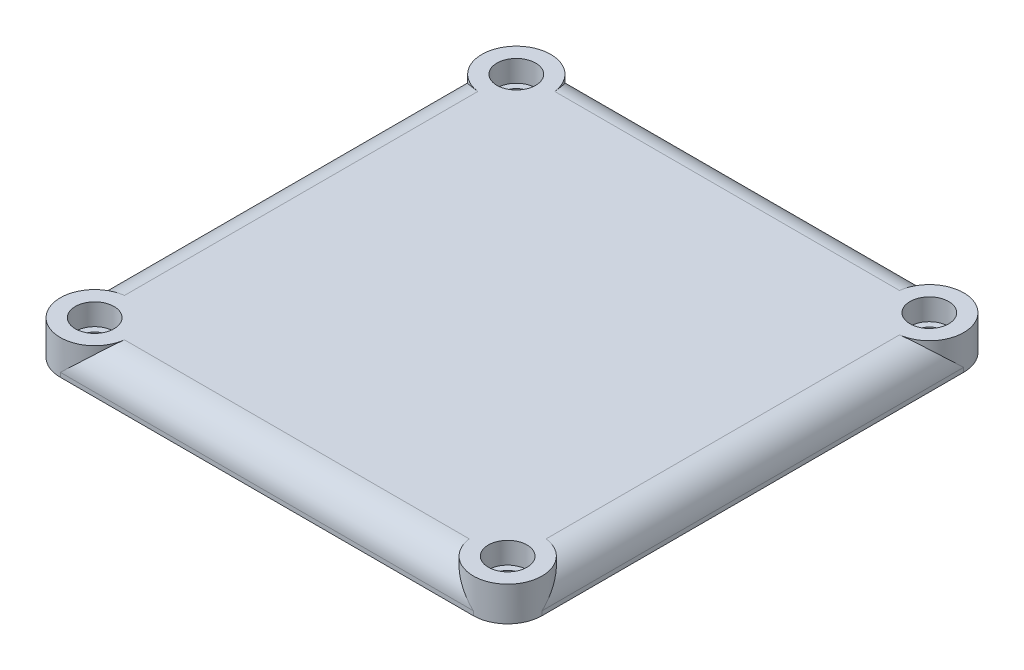
from build123d import *

# Parameters (mm, degrees)
BOSS_EXTRUDE1_DEPTH = 8
FILLET4_R           = 7
SKETCH2_R           = 7.999999999999998
SKETCH2_R_2         = 8.000000000000005
BOSS_EXTRUDE2_DEPTH = 8
CUT_EXTRUDE1_DEPTH  = 3
FILLET3_R           = 2
HOLE2_D             = 6
HOLE2_DEPTH         = 100
HOLE2_CBORE_D       = 9
HOLE2_CBORE_DEPTH   = 5


with BuildPart() as part:
    # Sketch1 → Boss-Extrude1 (new body)
    with BuildSketch(Plane(origin=(0, 0, 0), x_dir=(1, 0, 0), z_dir=(0, 1, 0))):
        with BuildLine():
            Line((-47.99999999999995, -57), (47.999999999999936, -57.000000000000014))
            ThreePointArc((47.999999999999936, -57.000000000000014), (53.656854249492376, -54.6568542494924), (55.99999999999999, -48.99999999999996))
            Line((55.99999999999999, -48.99999999999996), (56, 48.99999999999994))
            ThreePointArc((56, 48.99999999999994), (53.65685424949238, 54.65685424949238), (47.99999999999994, 57))
            Line((47.99999999999994, 57), (-47.99999999999996, 57))
            ThreePointArc((-47.99999999999996, 57), (-53.6568542494924, 54.65685424949238), (-56.000000000000014, 48.99999999999994))
            Line((-56.000000000000014, 48.99999999999994), (-56.00000000000001, -48.99999999999994))
            ThreePointArc((-56.00000000000001, -48.99999999999994), (-53.65685424949238, -54.65685424949238), (-47.99999999999995, -57))
        make_face()
    extrude(amount=BOSS_EXTRUDE1_DEPTH)

    # Fillet4
    fillet4_edges = [part.edges().sort_by_distance(p)[0] for p in [
        (53.65685424949238, 8, -54.65685424949238),
        (-7.11e-15, 8, -57),
        (-53.6568542494924, 8, -54.65685424949238),
        (-56.000000000000014, 8, 0),
        (-53.65685424949239, 8, 54.65685424949238),
        (-7.11e-15, 8, 57.00000000000001),
        (53.656854249492376, 8, 54.6568542494924),
        (55.99999999999999, 8, 7.11e-15),
    ]]
    fillet(fillet4_edges, radius=FILLET4_R)

    # Sketch2 → Boss-Extrude2 (add)
    with BuildSketch(Plane(origin=(0, 0, 0), x_dir=(-1, 0, 0), z_dir=(0, -1, 0))):
        with Locations((48.00000000000001, -49)):
            Circle(SKETCH2_R)
        with Locations((-47.99999999999999, -49.000000000000014)):
            Circle(SKETCH2_R_2)
        with Locations((-48, 49)):
            Circle(SKETCH2_R_2)
        with Locations((48.000000000000014, 49)):
            Circle(SKETCH2_R)
    extrude(amount=-BOSS_EXTRUDE2_DEPTH)

    # Sketch6 → Cut-Extrude1 (cut)
    with BuildSketch(Plane(origin=(0, 0, 0), x_dir=(-1, 0, 0), z_dir=(0, -1, 0))):
        with BuildLine():
            ThreePointArc((-48.99999999999984, -41.06274606680613), (-42.708497377870756, -42.99999999999998), (-40, -48.99999999999992))
            Line((-40.00000000000001, -49), (40.00000000000001, -49))
            ThreePointArc((40.00000000000001, -48.99999999999994), (42.70849737787087, -42.9999999999999), (49.00000000000012, -41.06274606680618))
            Line((48.99999999999999, -41.0627460668062), (48.99999999999999, 41.062746066806255))
            ThreePointArc((49.000000000000114, 41.062746066806234), (42.70849737787086, 42.999999999999964), (40.00000000000001, 49))
            Line((40.00000000000001, 49.00000000000001), (-39.999999999999936, 49.00000000000001))
            ThreePointArc((-39.999999999999936, 49.00000000000003), (-42.70849737787072, 43.00000000000006), (-48.99999999999983, 41.06274606680624))
            Line((-48.99999999999999, 41.06274606680623), (-48.99999999999999, -41.062746066806106))
        make_face()
    extrude(amount=-CUT_EXTRUDE1_DEPTH, mode=Mode.SUBTRACT)

    # Fillet3
    fillet3_edges = [part.edges().sort_by_distance(p)[0] for p in [
        (42.708497377870714, 3, -43.000000000000064),
        (-3.553e-14, 3, -49.00000000000001),
        (-48.99999999999999, 3, -2.842e-14),
        (-42.70849737787087, 3, 42.9999999999999),
        (42.708497377870756, 3, 42.99999999999998),
        (48.99999999999999, 3, -5.684e-14),
        (-42.70849737787086, 3, -42.99999999999996),
        (0, 3, 49),
    ]]
    fillet(fillet3_edges, radius=FILLET3_R)

    # Hole2
    with Locations(Plane(origin=(0, 8, 0), x_dir=(1, 0, 0), z_dir=(0, 1, 0))):
        with Locations((-48, 49), (48, 49), (-48, -49), (48, -49)):
            CounterBoreHole(HOLE2_D / 2, HOLE2_CBORE_D / 2, HOLE2_CBORE_DEPTH, depth=HOLE2_DEPTH)


solid = part.part
